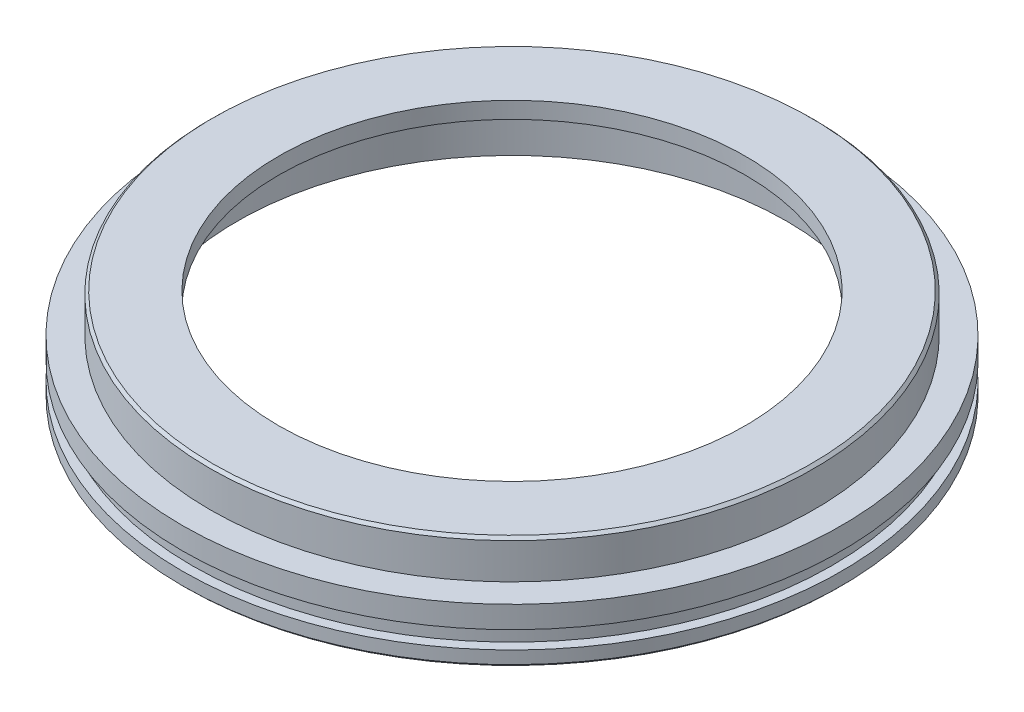
from build123d import *

# Parameters (mm, degrees)
SKETCH1_R           = 60
BOSS_EXTRUDE1_DEPTH = 10
SKETCH2_R           = 55
BOSS_EXTRUDE2_DEPTH = 7
SKETCH3_R           = 42.5
CUT_EXTRUDE1_DEPTH  = 87.539008545
SKETCH4_R           = 55
CUT_EXTRUDE2_DEPTH  = 3
SKETCH5_R           = 50
CUT_EXTRUDE3_DEPTH  = 11
SKETCH6_OUTSIDE_W   = 156.11
SKETCH6_OUTSIDE_H   = 156.11
SKETCH6_OUTSIDE_R   = 58.25
CUT_EXTRUDE4_DEPTH  = 3.2
CHAMFER1_SIZE       = 0.5
CHAMFER2_SIZE       = 0.5


with BuildPart() as part:
    # Sketch1 → Boss-Extrude1 (new body)
    with BuildSketch(Plane(origin=(0, 0, 0), x_dir=(1, 0, 0), z_dir=(0, 1, 0))):
        with Locations(Location((0, 0, 0), (0, 0, 270))):
            Circle(SKETCH1_R)
    extrude(amount=BOSS_EXTRUDE1_DEPTH)

    # Sketch2 → Boss-Extrude2 (add)
    with BuildSketch(Plane(origin=(0, 10, 0), x_dir=(1, 0, 0), z_dir=(0, 1, 0))):
        with Locations(Location((0, 0, 0), (0, 0, 270))):
            Circle(SKETCH2_R)
    extrude(amount=BOSS_EXTRUDE2_DEPTH)

    # Sketch3 → Cut-Extrude1 (cut, through all)
    with BuildSketch(Plane(origin=(0, 17, 0), x_dir=(1, 0, 0), z_dir=(0, 1, 0))):
        with Locations(Location((0, 0, 0), (0, 0, 270))):
            Circle(SKETCH3_R)
    extrude(amount=-CUT_EXTRUDE1_DEPTH, mode=Mode.SUBTRACT)

    # Sketch4 → Cut-Extrude2 (cut)
    with BuildSketch(Plane.XZ):
        with Locations(Location((0, 0, 0), (0, 0, 90))):
            Circle(SKETCH4_R)
    extrude(amount=-CUT_EXTRUDE2_DEPTH, mode=Mode.SUBTRACT)

    # Sketch5 → Cut-Extrude3 (cut)
    with BuildSketch(Plane.XZ.offset(-3)):
        with Locations(Location((0, 0, 0), (0, 0, 270))):
            Circle(SKETCH5_R)
    extrude(amount=-CUT_EXTRUDE3_DEPTH, mode=Mode.SUBTRACT)

    # Sketch6 outside → Cut-Extrude4 (cut)
    with BuildSketch(Plane(origin=(0, 6, 0), x_dir=(-1, 0, 0), z_dir=(0, -1, 0))):
        Rectangle(SKETCH6_OUTSIDE_W, SKETCH6_OUTSIDE_H)
        with Locations(Location((0, 0, 0), (0, 0, 90))):
            Circle(SKETCH6_OUTSIDE_R, mode=Mode.SUBTRACT)
    extrude(amount=CUT_EXTRUDE4_DEPTH, mode=Mode.SUBTRACT)

    # Chamfer1
    chamfer1_edges = [part.edges().sort_by_distance(p)[0] for p in [
        (0, 0, -60),
    ]]
    chamfer(chamfer1_edges, length=CHAMFER1_SIZE)

    # Chamfer2
    chamfer2_edges = [part.edges().sort_by_distance(p)[0] for p in [
        (0, 17, -55),
    ]]
    chamfer(chamfer2_edges, length=CHAMFER2_SIZE)


solid = part.part
